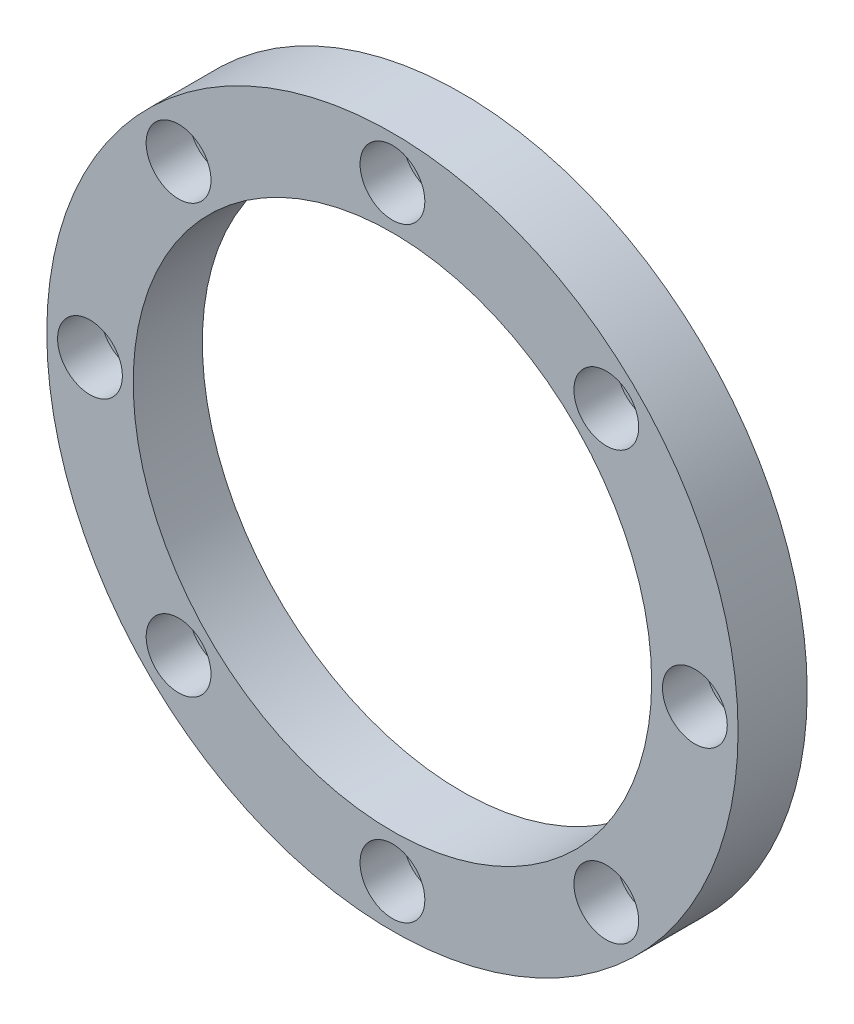
from build123d import *

# Parameters (mm, degrees)
SKETCH1_R                                            = 40
SKETCH1_R_2                                          = 30
BOSS_EXTRUDE1_DEPTH                                  = 4
HOLE_SIZE_BY_SOCKET_HEAD_CAP_SCREW_TYPE1_D           = 4.2
HOLE_SIZE_BY_SOCKET_HEAD_CAP_SCREW_TYPE1_CBORE_D     = 7.5
HOLE_SIZE_BY_SOCKET_HEAD_CAP_SCREW_TYPE1_CBORE_DEPTH = 5
CIRPATTERN1_COUNT                                    = 8


with BuildPart() as part:
    # Sketch1 → Boss-Extrude1 (new, symmetric)
    with BuildSketch(Plane.XY):
        Circle(SKETCH1_R)
        Circle(SKETCH1_R_2, mode=Mode.SUBTRACT)
    extrude(amount=BOSS_EXTRUDE1_DEPTH, both=True)

    # Hole Size by Socket Head Cap Screw Type1 (through all)
    with Locations(Plane.XY.offset(4)):
        with Locations((35, 0)):
            hole_size_by_socket_head_cap_screw_type1 = CounterBoreHole(HOLE_SIZE_BY_SOCKET_HEAD_CAP_SCREW_TYPE1_D / 2, HOLE_SIZE_BY_SOCKET_HEAD_CAP_SCREW_TYPE1_CBORE_D / 2, HOLE_SIZE_BY_SOCKET_HEAD_CAP_SCREW_TYPE1_CBORE_DEPTH)

    # CirPattern1: Hole Size by Socket Head Cap Screw Type1 ×8 about axis
    cirpattern1_axis = Axis((0, 0, 0), (0, 0, 1))
    for i in range(1, CIRPATTERN1_COUNT):
        add(hole_size_by_socket_head_cap_screw_type1.rotate(cirpattern1_axis, i * 360 / CIRPATTERN1_COUNT), mode=Mode.SUBTRACT)


solid = part.part
